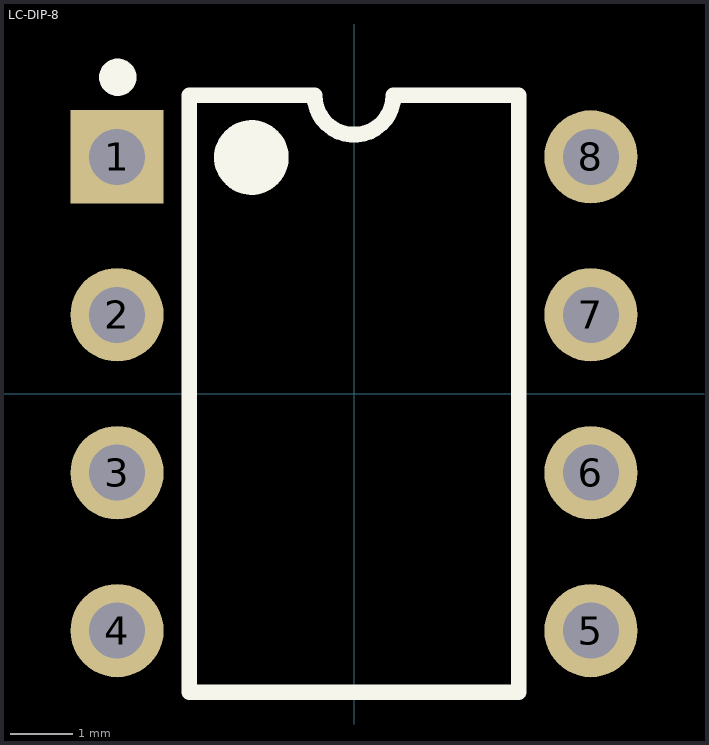
[diagram p0: the footprint, top view; thin cyan lines are the x and y axes]
# Altium footprint library MISC86340-9.PcbLib: 1 footprints
Each footprint in its own frame and in the unit in brackets; x right, y up, seen from the top. Pads: shape width x height; smd on the part's side, far side on the other; paste and mask are expansions set on the pad; w line width, h text height; cw(c..) or ccw(c..) is an arc to the next point about the centre after c.

## LC-DIP-8 [mm]
pads (8):
  rect 1.5x1.5 hole 0.9: 1(-3.81,3.81)
  round 1.5 hole 0.9: 2(-3.81,1.27) 3(-3.81,-1.27) 4(-3.81,-3.81) 5(3.81,-3.81) 6(3.81,-1.27) 7(3.81,1.27) 8(3.81,3.81)
Top Overlay:
  circle w0.6: c-1.65,3.8 r0.3
  circle w0.3: c-3.8,5.09 r0.15
  lines w0.254: -2.65,-4.8 2.65,-4.8 2.65,4.8 0.635,4.8 cw(c0,4.8) -0.635,4.8 -2.65,4.8 -2.65,-4.8
3D body "SW3dPS-DIP08-300.STEP": height 5.08, standoff -2.49, extent -3.935,-5.46 3.935,5.46